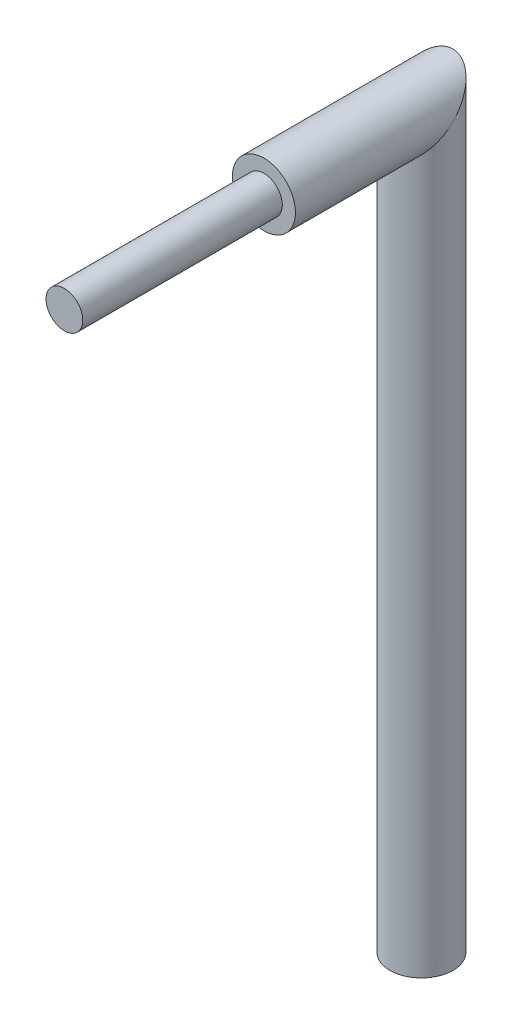
SolidWorks part; units mm, degrees
material "AISI 304"
ref_plane "Front Plane" through (0, 0, 0) normal (0, 0, 1) x (1, 0, 0)
ref_plane "Top Plane" through (0, 0, 0) normal (0, 1, 0) x (1, 0, 0)
ref_plane "Right Plane" through (0, 0, 0) normal (1, 0, 0) x (0, 0, -1)
sketch "Sketch1" plane through (0, 0, 0) normal (0, 1, 0) x (1, 0, 0)
  circle A0 centre (0, 0) radius 3
  dimension "D1" = 6
extrude "Boss-Extrude1" add sketch "Sketch1" along normal blind 70
sketch "Sketch3" plane through (0, 0, 0) normal (0, 0, 1) x (1, 0, 0)
  line L0 (3, 70) -> (-3, 70) construction
  circle A0 centre (0, 70) radius 3
extrude "Boss-Extrude3" add sketch "Sketch3" along normal blind 15
sketch "Sketch4" plane through (0, 70, 0) normal (0, 1, 0) x (1, 0, 0)
  line L0 (-3, 0) -> (3, 0) construction
  line L1 (-3, 0) -> (3, 0)
  arc A0 (3, 0) -> (-3, 0) centre (0, 0) ccw construction
  arc A1 (3, 0) -> (-3, 0) centre (0, 0) ccw
extrude "Boss-Extrude4" add sketch "Sketch4" along normal blind 4
sketch "Sketch5" plane through (0, 0, 15) normal (0, 0, 1) x (1, 0, 0)
  line L0 (-3, 74) -> (-3, 70) construction
  line L2 (-3, 70) -> (-3, 74)
  line L3 (-3, 74) -> (3, 74)
  line L4 (3, 70) -> (3, 74)
  line L5 (-0.12, 69.84) -> (3, 74) construction
  line L6 (-3, 74) -> (-1.08, 71.44) construction
  arc A0 (3, 70) -> (-3, 70) centre (0, 70) ccw
  circle A1 centre (0, 70) radius 3 construction
extrude "Cut-Extrude1" cut sketch "Sketch5" against normal through all
sketch "Sketch6" plane through (0, 0, 15) normal (0, 0, 1) x (1, 0, 0)
  circle A0 centre (0, 70) radius 1.75
  dimension "D1" = 3.5
extrude "Boss-Extrude5" add sketch "Sketch6" along normal blind 19
